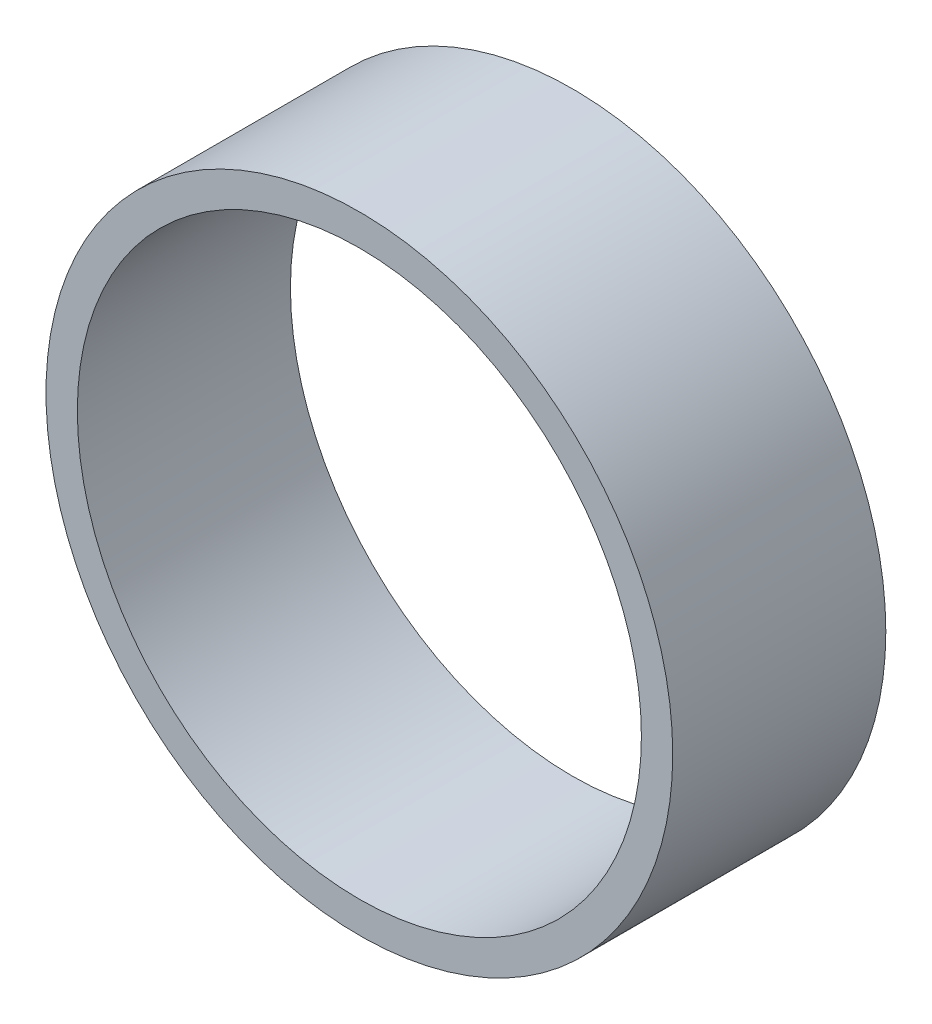
SolidWorks part; units mm, degrees
ref_plane "前视基准面" through (0, 0, 0) normal (0, 0, 1) x (1, 0, 0)
ref_plane "上视基准面" through (0, 0, 0) normal (0, 1, 0) x (1, 0, 0)
ref_plane "右视基准面" through (0, 0, 0) normal (1, 0, 0) x (0, 0, -1)
other "Configuration Table"
sketch "草图1" plane through (0, 0, 0) normal (0, 0, 1) x (1, 0, 0)
  circle A0 centre (0, 0) radius 50
  circle A1 centre (0, 0) radius 45
  dimension "D1" = 90
  dimension "D2" = 100
extrude "凸台-拉伸1" add sketch "草图1" along normal blind 34
